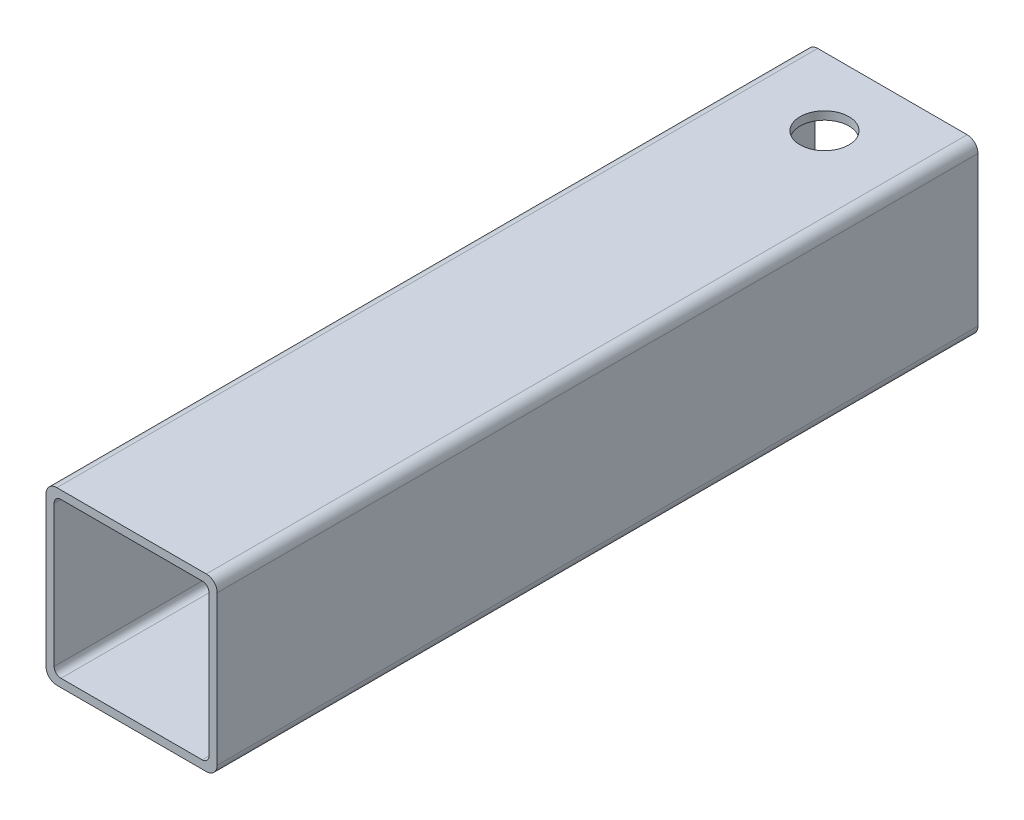
SolidWorks part; units mm, degrees
ref_plane "Front Plane" through (0, 0, 0) normal (0, 0, 1) x (1, 0, 0)
ref_plane "Top Plane" through (0, 0, 0) normal (0, 1, 0) x (1, 0, 0)
ref_plane "Right Plane" through (0, 0, 0) normal (1, 0, 0) x (0, 0, -1)
sketch "Sketch1" plane through (0, 0, 0) normal (0, 0, 1) x (1, 0, 0)
  line L1 (0, 0) -> (126, 0)
  line L2 (0, 0) -> (0, 126)
  line L3 (0, 126) -> (126, 126)
  line L4 (126, 0) -> (126, 126)
  line L5 (6, 120) -> (120, 120)
  line L6 (6, 120) -> (6, 6)
  line L7 (6, 6) -> (120, 6)
  line L8 (120, 120) -> (120, 6)
  dimension "D1" = 126
  dimension "D2" = 126
  dimension "D3" = 6
  dimension "D4" = 6
  dimension "D5" = 6
  dimension "D6" = 6
extrude "Boss-Extrude1" add sketch "Sketch1" along normal blind 560
fillet "Fillet1" radius 8 4 edges at (126, 0, 280) (0, 0, 280) (0, 126, 280) (126, 126, 280)
fillet "Fillet2" radius 5 4 edges at (6, 6, 280) (120, 6, 280) (120, 120, 280) (6, 120, 280)
sketch "Sketch3" plane through (0, 0, 0) normal (0, -1, 0) x (1, 0, 0)
  line L0 (63, 0) -> (63, 560) construction
  line L1 (8, 0) -> (118, 0) construction
  line L2 (8, 560) -> (118, 560) construction
  circle A0 centre (63, 50) radius 18
  dimension "D1" = 50
  dimension "D2" = 36
extrude "Cut-Extrude1" cut sketch "Sketch3" against normal blind 260
sketch "Sketch4" [suppressed] plane through (0, 0, 0) normal (0, 0, -1) x (-1, 0, 0)
  line L0 (-63, 126) -> (-63, 0)
  line L1 (-116, 126) -> (-10, 126) construction
  line L2 (-10, 0) -> (-116, 0) construction
